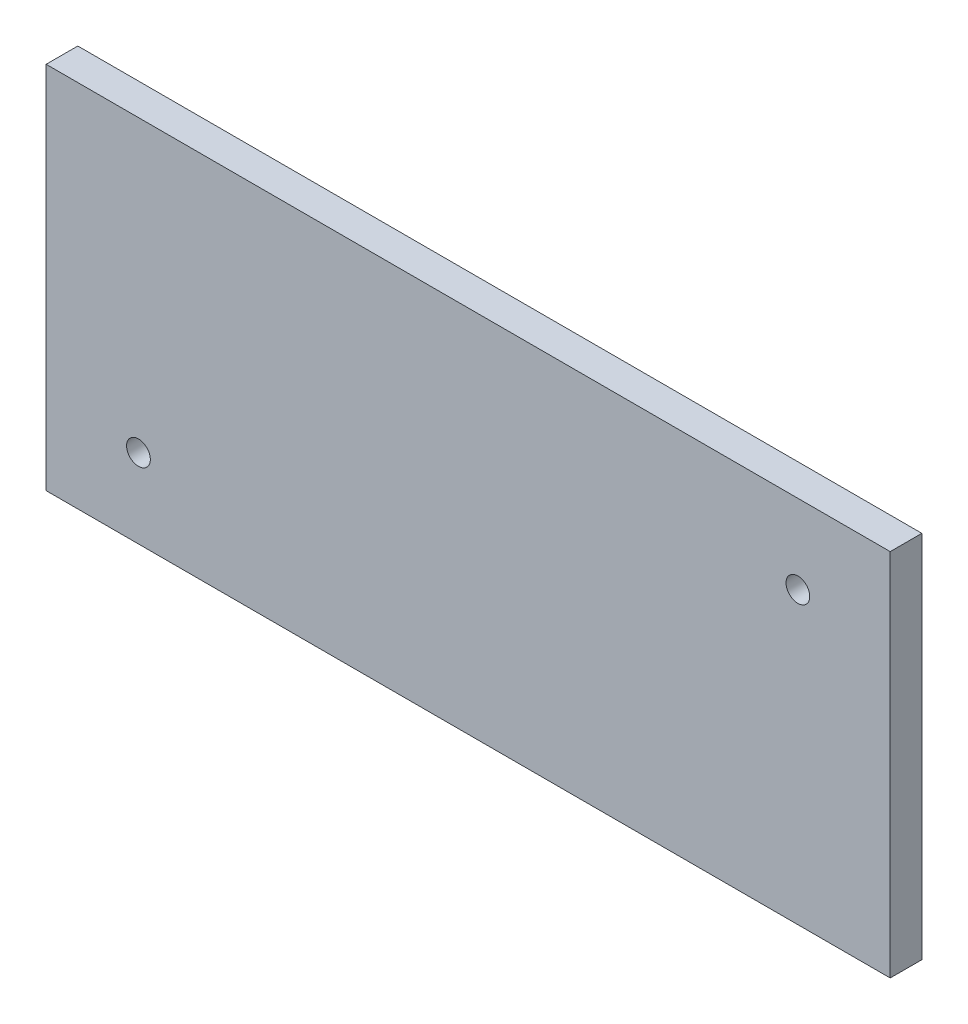
SolidWorks part; units mm, degrees
ref_plane "前视基准面" through (0, 0, 0) normal (0, 0, 1) x (1, 0, 0)
ref_plane "上视基准面" through (0, 0, 0) normal (0, 1, 0) x (1, 0, 0)
ref_plane "右视基准面" through (0, 0, 0) normal (1, 0, 0) x (0, 0, -1)
other "Configuration Table"
sketch "草图1" plane through (0, 0, 0) normal (0, 0, 1) x (1, 0, 0)
  line L0 (-160, -70) -> (160, -70)
  line L1 (160, -70) -> (160, 70)
  line L2 (160, 70) -> (-160, 70)
  line L3 (-160, 70) -> (-160, -70)
  point P0 (0, 0)
  dimension "D1" = 160
  dimension "D2" = 320
  dimension "D3" = 70
  dimension "D4" = 140
extrude "凸台-拉伸1" add sketch "草图1" against normal mid plane 12
sketch "草图2" plane through (0, 0, 0) normal (0, 0, 1) x (1, 0, 0)
  circle A0 centre (-125, -40) radius 4.5
  circle A1 centre (125, 40) radius 4.5
  point P0 (0, 0)
  dimension "D1" = 9
  dimension "D2" = 9
  dimension "D3" = 125
  dimension "D4" = 250
  dimension "D5" = 40
  dimension "D6" = 80
extrude "切除-拉伸1" cut sketch "草图2" against normal mid plane 32
